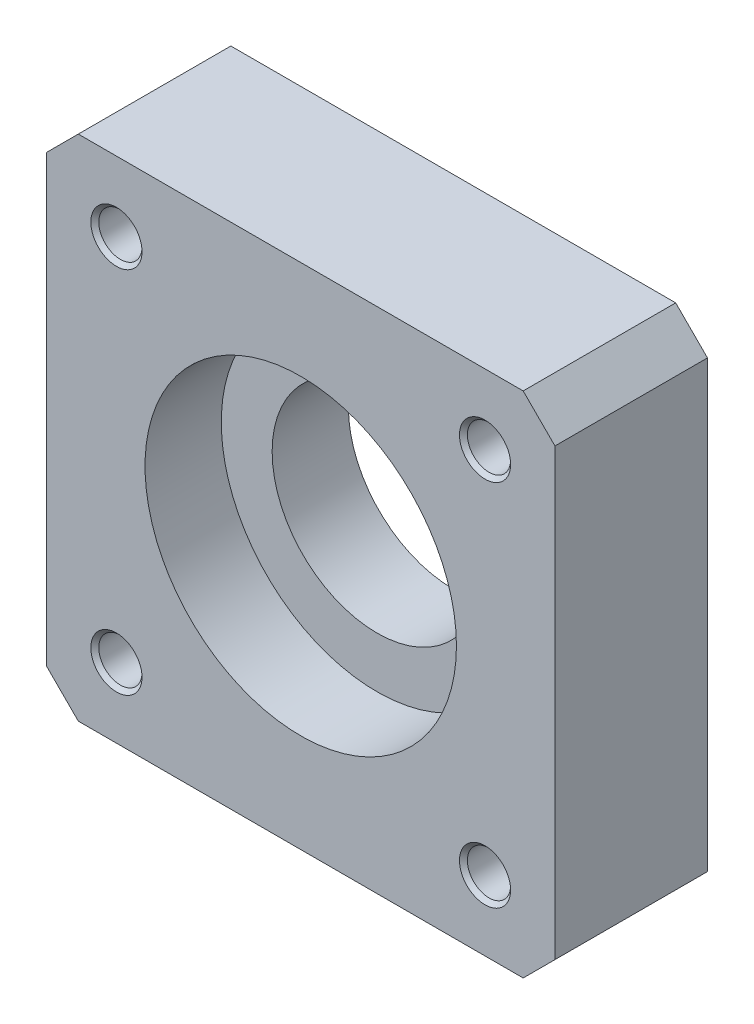
from build123d import *

# Parameters (mm, degrees)
SKETCH1_W                   = 80
SKETCH1_H                   = 80
BOSS_EXTRUDE1_DEPTH         = 24
HOLE1_D                     = 33
HOLE1_CBORE_D               = 49
HOLE1_CBORE_DEPTH           = 12
M8_TAPPED_HOLE1_D           = 6.8
M8_TAPPED_HOLE1_CSINK_D     = 8.05
M8_TAPPED_HOLE1_CSINK_ANGLE = 90
CHAMFER1_SIZE               = 5


with BuildPart() as part:
    # Sketch1 → Boss-Extrude1 (new body)
    with BuildSketch(Plane.XY):
        with Locations((-12.568836811, 18.618181818)):
            Rectangle(SKETCH1_W, SKETCH1_H)
    extrude(amount=BOSS_EXTRUDE1_DEPTH)

    # Hole1 (through all)
    with Locations(Plane.XY.offset(24)):
        with Locations((-12.568836811, 18.618181818)):
            CounterBoreHole(HOLE1_D / 2, HOLE1_CBORE_D / 2, HOLE1_CBORE_DEPTH)

    # M8 Tapped Hole1 (through all)
    with Locations(Plane.XY.offset(24)):
        with Locations((-41.568836811, 47.618181818), (16.431163189, 47.618181818), (16.431163189, -10.381818182), (-41.568836811, -10.381818182)):
            CounterSinkHole(M8_TAPPED_HOLE1_D / 2, M8_TAPPED_HOLE1_CSINK_D / 2, counter_sink_angle=M8_TAPPED_HOLE1_CSINK_ANGLE)

    # Chamfer1
    chamfer1_edges = [part.edges().sort_by_distance(p)[0] for p in [
        (-52.568836811, 58.618181818, 12),
        (27.431163189, 58.618181818, 12),
        (27.431163189, -21.381818182, 12),
        (-52.568836811, -21.381818182, 12),
    ]]
    chamfer(chamfer1_edges, length=CHAMFER1_SIZE)


solid = part.part
